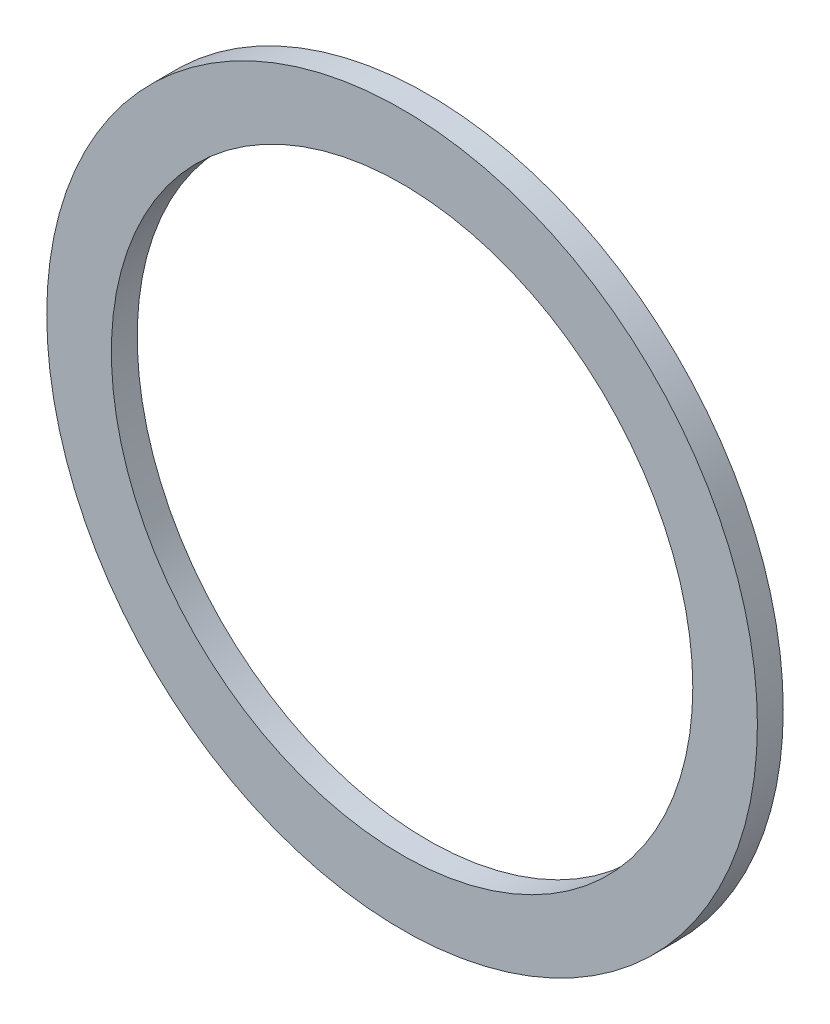
from build123d import *

# Parameters (mm, degrees)
SKETCH_1_R      = 27.5
SKETCH_1_R_2    = 22.5
EXTRUDE_1_DEPTH = 2


with BuildPart() as part:
    # 草图1 → 凸台-拉伸1 (new body)
    with BuildSketch(Plane.XY):
        Circle(SKETCH_1_R)
        Circle(SKETCH_1_R_2, mode=Mode.SUBTRACT)
    extrude(amount=EXTRUDE_1_DEPTH)


solid = part.part
